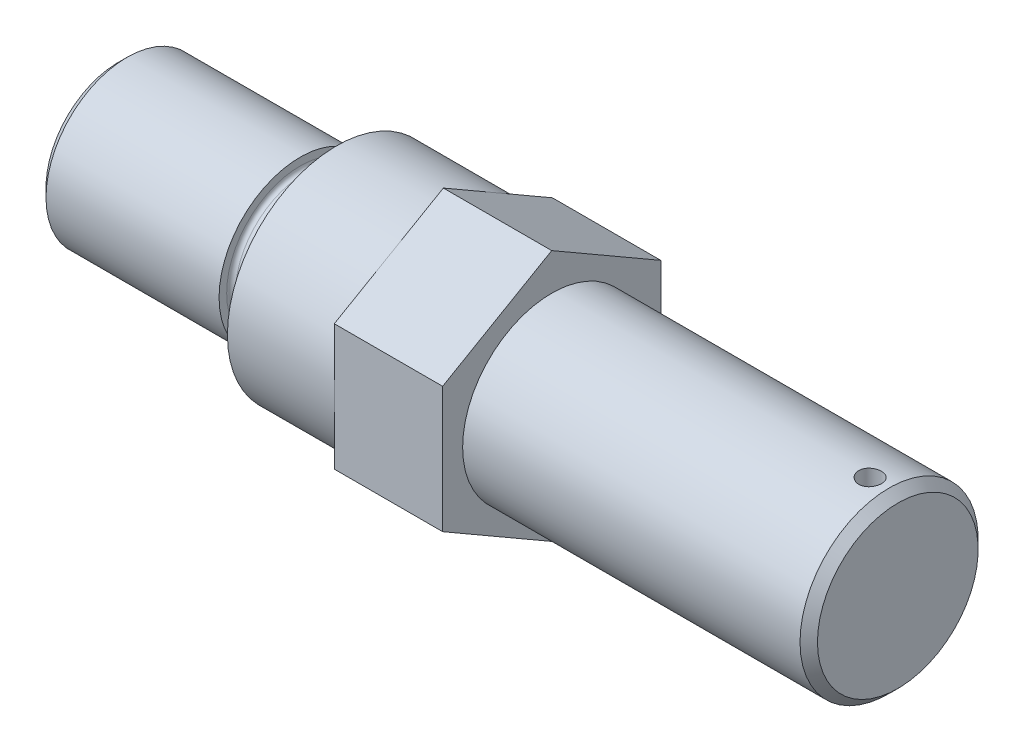
from build123d import *

# Parameters (mm, degrees)
CHAMFER1_SIZE       = 1.524
BOSS_EXTRUDE1_DEPTH = 18.923
FILLET1_R           = 0.762
SKETCH3_R           = 1.98435
CUT_EXTRUDE1_DEPTH  = 25


with BuildPart() as part:
    # Sketch1 → Revolve1 (revolve)
    with BuildSketch(Plane.XY, mode=Mode.PRIVATE) as revolve1_sk:
        Polygon((0, 0), (0, 14.1605), (31.75, 14.1605), (31.75, 12.065), (38.1, 12.065), (38.1, 19.05), (75.692, 19.05), (75.692, 15.5575), (136.144, 15.5575), (136.144, 0), align=None)
    revolve(revolve1_sk.sketch.rotate(Axis((0, 0, 0), (1, 0, 0)), 90), axis=Axis((0, 0, 0), (1, 0, 0)))

    # Chamfer1
    chamfer1_edges = [part.edges().sort_by_distance(p)[0] for p in [
        (0, 0, -14.1605),
        (136.144, 0, -15.5575),
    ]]
    chamfer(chamfer1_edges, length=CHAMFER1_SIZE)

    # Sketch2 → Boss-Extrude1 (add)
    with BuildSketch(Plane(origin=(75.692, 0, 0), x_dir=(0, 0, -1), z_dir=(1, 0, 0))):
        Polygon((0, 21.997045256), (-19.05, 10.998522628), (-19.05, -10.998522628), (0, -21.997045256), (19.05, -10.998522628), (19.05, 10.998522628), align=None)
    extrude(amount=-BOSS_EXTRUDE1_DEPTH)

    # Fillet1
    fillet1_edges = [part.edges().sort_by_distance(p)[0] for p in [
        (38.1, 0, -12.065),
        (31.75, 0, -12.065),
    ]]
    fillet(fillet1_edges, radius=FILLET1_R)

    # Sketch3 → Cut-Extrude1 (cut, symmetric)
    with BuildSketch(Plane(origin=(0, 0, 0), x_dir=(1, 0, 0), z_dir=(0, 1, 0))):
        with Locations(Location((131.318, 0, 0), (0, 0, 270))):
            Circle(SKETCH3_R)
    extrude(amount=CUT_EXTRUDE1_DEPTH, both=True, mode=Mode.SUBTRACT)


solid = part.part
